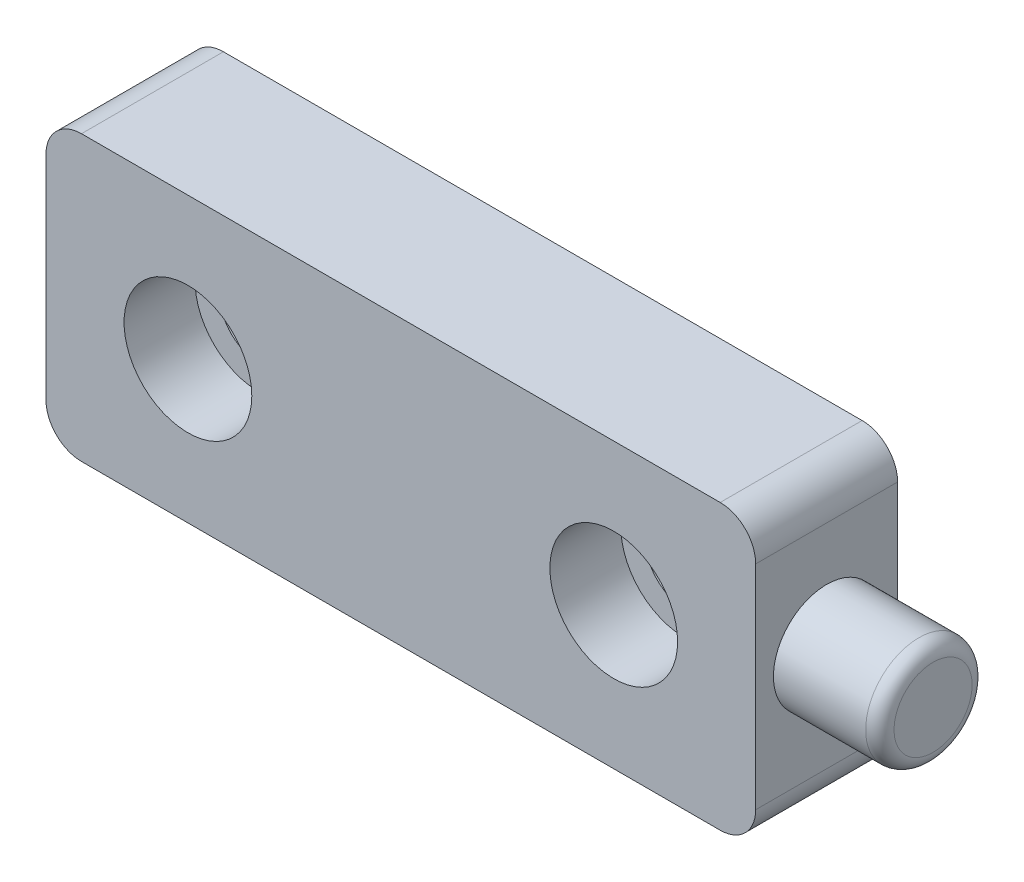
from build123d import *

# Parameters (mm, degrees)
SKETCH1_W           = 100
SKETCH1_H           = 40
SKETCH1_R           = 5.5
BOSS_EXTRUDE1_DEPTH = 10
SKETCH2_R           = 7.5
BOSS_EXTRUDE2_DEPTH = 15
FILLET1_R           = 2
SKETCH3_R           = 9
CUT_EXTRUDE1_DEPTH  = 10
FILLET2_R           = 5


with BuildPart() as part:
    # Sketch1 → Boss-Extrude1 (new, symmetric)
    with BuildSketch(Plane.XY):
        Rectangle(SKETCH1_W, SKETCH1_H)
        with Locations((-30, 0)):
            Circle(SKETCH1_R, mode=Mode.SUBTRACT)
        with Locations((30, 0)):
            Circle(SKETCH1_R, mode=Mode.SUBTRACT)
    extrude(amount=BOSS_EXTRUDE1_DEPTH, both=True)

    # Sketch2 → Boss-Extrude2 (add)
    with BuildSketch(Plane(origin=(50, 0, 0), x_dir=(0, 0, -1), z_dir=(1, 0, 0))):
        Circle(SKETCH2_R)
    extrude(amount=BOSS_EXTRUDE2_DEPTH)

    # Fillet1
    fillet1_edges = [part.edges().sort_by_distance(p)[0] for p in [
        (65, 0, 7.5),
    ]]
    fillet(fillet1_edges, radius=FILLET1_R)

    # Sketch3 → Cut-Extrude1 (cut)
    with BuildSketch(Plane.XY.offset(10)):
        with Locations((-30, 0)):
            Circle(SKETCH3_R)
        with Locations((30, 0)):
            Circle(SKETCH3_R)
    extrude(amount=-CUT_EXTRUDE1_DEPTH, mode=Mode.SUBTRACT)

    # Fillet2
    fillet2_edges = [part.edges().sort_by_distance(p)[0] for p in [
        (50, -20, 0),
        (-50, -20, 0),
        (-50, 20, 0),
        (50, 20, 0),
    ]]
    fillet(fillet2_edges, radius=FILLET2_R)


solid = part.part
